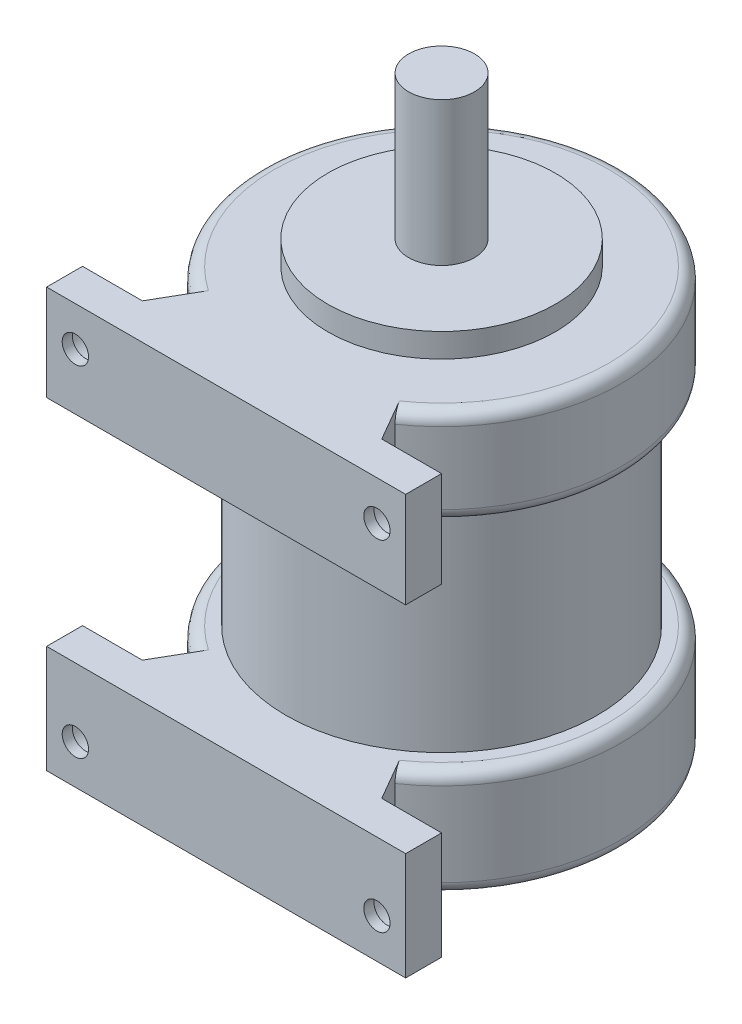
SolidWorks part; units mm, degrees
ref_plane "前视基准面" through (0, 0, 0) normal (0, 0, 1) x (1, 0, 0)
ref_plane "上视基准面" through (0, 0, 0) normal (0, 1, 0) x (1, 0, 0)
ref_plane "右视基准面" through (0, 0, 0) normal (1, 0, 0) x (0, 0, -1)
sketch "草图1" plane through (0, 0, 0) normal (0, 1, 0) x (1, 0, 0)
  circle A0 centre (0, 0) radius 150
  dimension "D1" = 300
extrude "凸台-拉伸1" add sketch "草图1" along normal blind 350
sketch "草图2" plane through (0, 0, 0) normal (0, -1, 0) x (1, 0, 0)
  line L0 (0, 0) -> (0, -50000) construction
  line L1 (-84.8234, 123.7133) -> (-100, 150)
  line L2 (-100, 150) -> (-150, 150)
  line L3 (-150, 150) -> (-150, 180)
  line L4 (-150, 180) -> (150, 180)
  line L5 (150, 150) -> (150, 180)
  line L6 (100, 150) -> (150, 150)
  line L7 (84.8234, 123.7133) -> (100, 150)
  circle A0 centre (0, 0) radius 150 construction
  arc A1 (84.8234, 123.7133) -> (-84.8234, 123.7133) centre (0, 0) ccw
  point P11 (0, 180)
  dimension "D1" = 150
  dimension "D2" = 30
  dimension "D3" = 180
  dimension "D4" = 60
  dimension "D5" = 50
extrude "凸台-拉伸2" add sketch "草图2" against normal blind 350
sketch "草图3" plane through (0, 350, 0) normal (0, 1, 0) x (1, 0, 0)
  circle A0 centre (0, 0) radius 95
  dimension "D1" = 190
extrude "凸台-拉伸3" add sketch "草图3" along normal blind 20
sketch "草图4" plane through (0, 350, 0) normal (0, 1, 0) x (1, 0, 0)
  circle A0 centre (0, 0) radius 130
  dimension "270" = 260
extrude "切除-拉伸1" cut sketch "草图4" against normal blind 180 from offset 80 flip side to cut offset against normal yes
fillet "圆角1" radius 10 4 edges at (0, 0, -150) (0, 90, -150) (0, 270, -150) (0, 350, -150)
sketch "草图5" plane through (0, 370, 0) normal (0, 1, 0) x (1, 0, 0)
  circle A0 centre (0, 0) radius 27.5
  dimension "D1" = 55
extrude "凸台-拉伸4" add sketch "草图5" along normal blind 120 separate body
hole_wizard "打孔尺寸(%根据)内六角圆柱头螺钉的类型1" positions "草图6" profile "草图7" counterbore size "M20" standard "GB" end condition through all
sketch "草图6" plane through (0, 0, 150) normal (0, 0, -1) x (-1, 0, 0)
  line L0 (150, 280) -> (150, 340) construction
  line L1 (-150, 340) -> (-150, 280) construction
  line L2 (140, 350) -> (-140, 350) construction
  line L3 (-140, 0) -> (140, 0) construction
  point P0 (-126, 317)
  point P2 (-126, 33)
  point P4 (126, 33)
  point P6 (126, 317)
  dimension "D1" = 24
  dimension "D2" = 24
  dimension "D3" = 33
  dimension "D4" = 33
sketch "草图7" plane through (126, 317, 150) normal (1, 0, 0) x (0, 1, 0)
  line L0 (0, 0) -> (0, 30)
  line L1 (0, 30) -> (11, 30)
  line L3 (11, 30) -> (11, 21.5)
  line L4 (11, 21.5) -> (16.5, 21.5)
  line L5 (16.5, 21.5) -> (16.5, 0)
  line L7 (16.5, 0) -> (0, 0)
  line L11 (0, -6.35) -> (0, 107.95) construction
  dimension "通孔孔直径" = 22
  dimension "通孔孔深度" = 30
  dimension "柱形沉头孔直径" = 33
  dimension "柱形沉头孔深度" = 21.5
